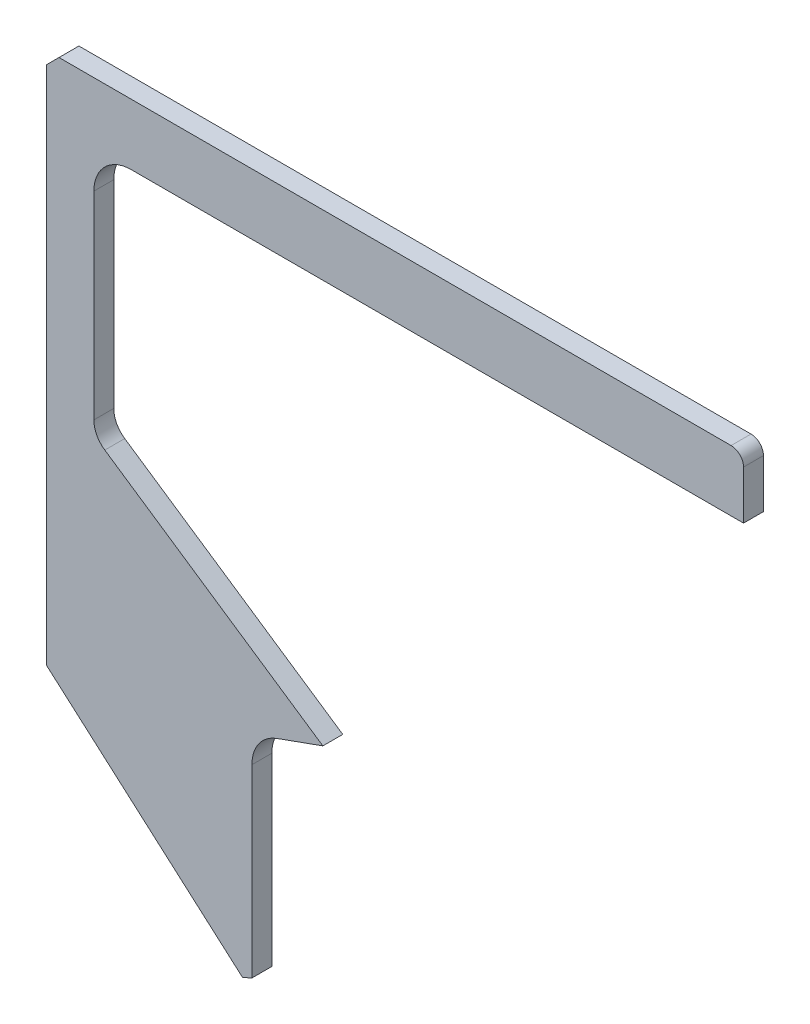
from build123d import *

# Parameters (mm, degrees)
BOSS_EXTRUDE1_DEPTH = 16


with BuildPart() as part:
    # Sketch1 → Boss-Extrude1 (new body)
    with BuildSketch(Plane.XY):
        with BuildLine():
            Line((0, 145), (0, 563))
            Line((0, 563), (10, 573))
            Line((10, 573), (550, 573))
            ThreePointArc((550, 573), (557.071067812, 570.071067812), (560, 563))
            Line((560, 563), (560, 524))
            Line((560, 524), (68, 524))
            ThreePointArc((68, 524), (46.786796564, 515.213203436), (38, 494))
            Line((38, 494), (38, 334.829857024))
            ThreePointArc((38, 334.829857024), (40.33946289, 325.443407802), (46.8105429, 318.252883543))
            Line((46.8105429, 318.252883543), (222, 200))
            Line((222, 200), (184.847185197, 186.638022746))
            ThreePointArc((184.847185197, 186.638022746), (170.458357389, 175.662455442), (165, 158.408245001))
            Line((165, 158.408245001), (165, 10))
            Line((165, 10), (157.488351016, 6.601146077))
            Line((157.488351016, 6.601146077), (0, 145))
        make_face()
    extrude(amount=BOSS_EXTRUDE1_DEPTH)


solid = part.part
